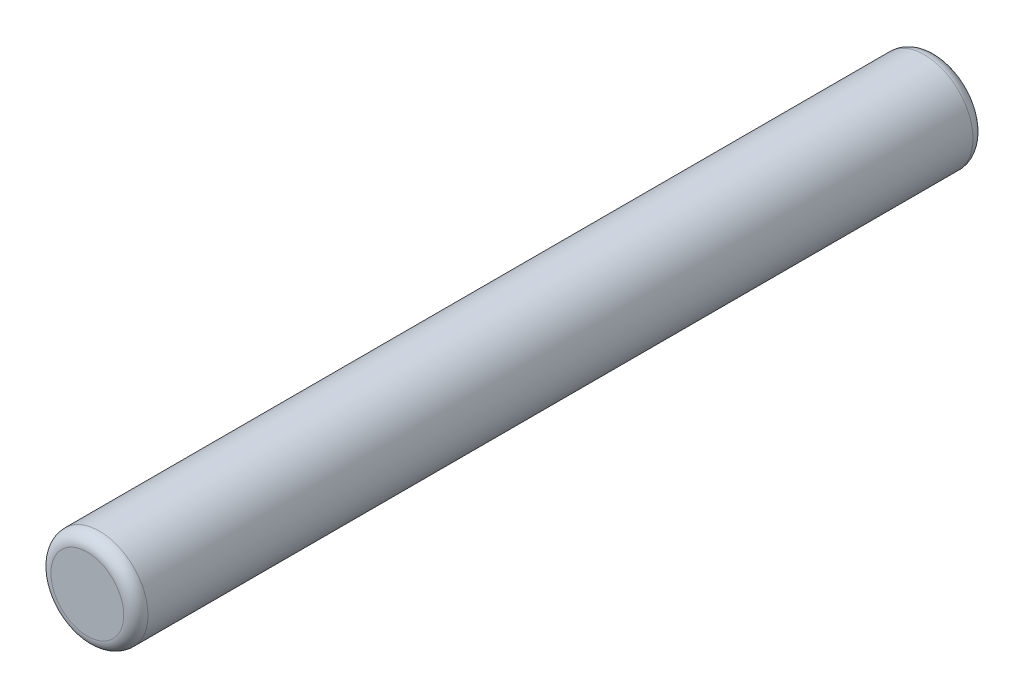
from build123d import *

# Parameters (mm, degrees)
SKETCH1_R           = 2
BOSS_EXTRUDE1_DEPTH = 35
FILLET1_R           = 0.5


with BuildPart() as part:
    # Sketch1 → Boss-Extrude1 (new body)
    with BuildSketch(Plane.XY):
        Circle(SKETCH1_R)
    extrude(amount=BOSS_EXTRUDE1_DEPTH)

    # Fillet1
    fillet1_edges = [part.edges().sort_by_distance(p)[0] for p in [
        (-2, 0, 0),
        (-2, 0, 35),
    ]]
    fillet(fillet1_edges, radius=FILLET1_R)


solid = part.part
